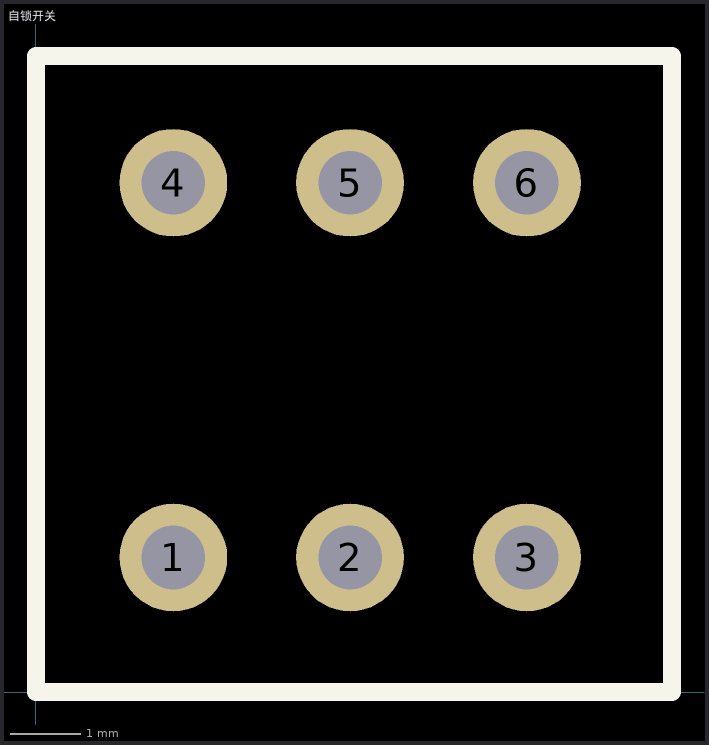
[diagram p0: the footprint, top view; thin cyan lines are the x and y axes]
# Altium footprint library MISC86340-30.PcbLib: 1 footprints
Each footprint in its own frame and in the unit in brackets; x right, y up, seen from the top. Pads: shape width x height; smd on the part's side, far side on the other; paste and mask are expansions set on the pad; w line width, h text height; cw(c..) or ccw(c..) is an arc to the next point about the centre after c.

## 自锁开关 [mm]
pads (6):
  round 1.524 hole 0.9: 1(1.945,1.905) 2(4.445,1.905) 3(6.945,1.905) 4(1.945,7.205) 5(4.445,7.205) 6(6.945,7.205)
Top Overlay:
  lines w0.254: 0,0 0,9 9,9 9,0 0,0